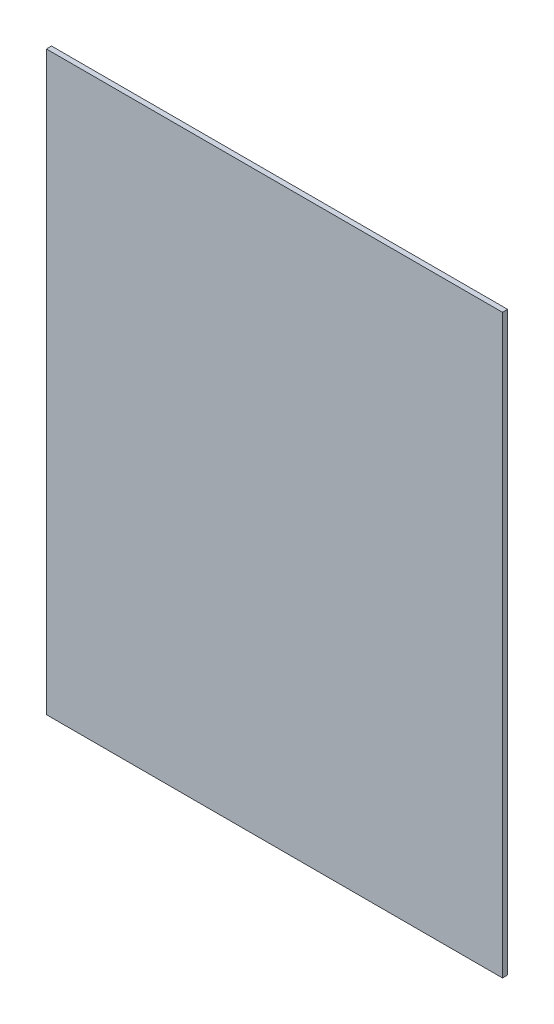
from build123d import *

# Parameters (mm, degrees)
SKETCH_1_W      = 356
SKETCH_1_H      = 450
EXTRUDE_1_DEPTH = 4


with BuildPart() as part:
    # 草图1 → 凸台-拉伸1 (new body)
    with BuildSketch(Plane.XY):
        Rectangle(SKETCH_1_W, SKETCH_1_H)
    extrude(amount=EXTRUDE_1_DEPTH)


solid = part.part
